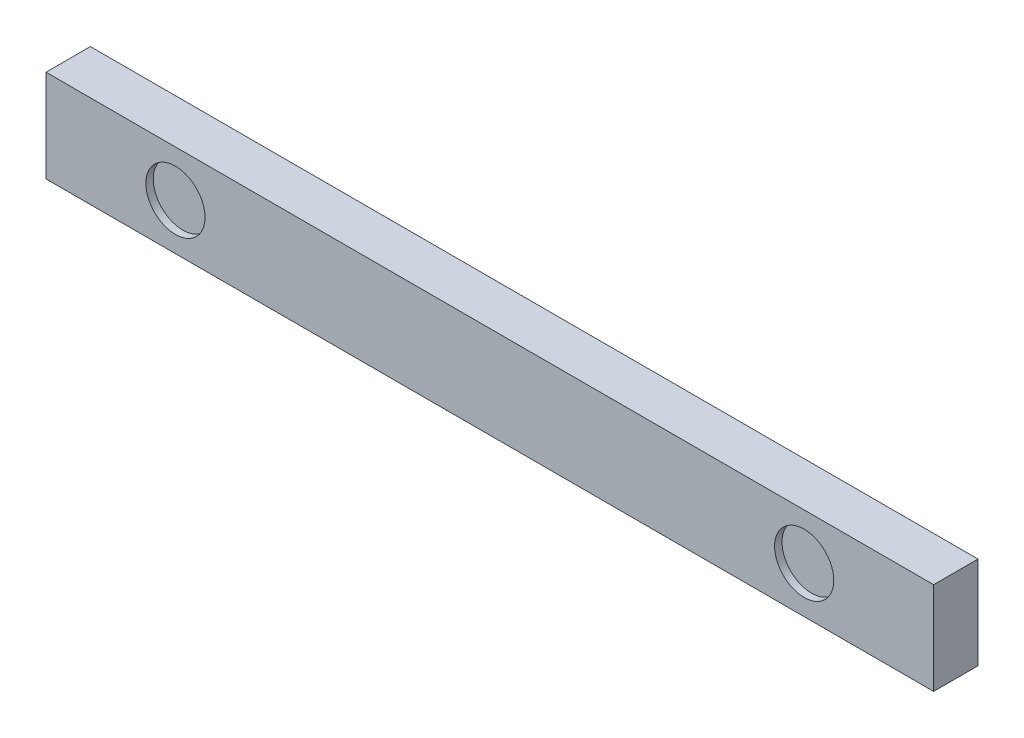
SolidWorks part; units mm, degrees
ref_plane "前视基准面" through (0, 0, 0) normal (0, 0, 1) x (1, 0, 0)
ref_plane "上视基准面" through (0, 0, 0) normal (0, 1, 0) x (1, 0, 0)
ref_plane "右视基准面" through (0, 0, 0) normal (1, 0, 0) x (0, 0, -1)
sketch "草图1" plane through (0, 0, 0) normal (0, 0, 1) x (1, 0, 0)
  line L1 (-120, -12.5) -> (120, -12.5)
  line L2 (-120, -12.5) -> (-120, 12.5)
  line L3 (-120, 12.5) -> (120, 12.5)
  line L4 (120, -12.5) -> (120, 12.5)
  line L5 (-120, -12.5) -> (120, 12.5) construction
  line L6 (-120, 12.5) -> (120, -12.5) construction
  point P0 (0, 0)
  dimension "D1" = 25
  dimension "D2" = 240
extrude "凸台-拉伸1" add sketch "草图1" along normal blind 12
sketch "草图2" plane through (0, 0, 12) normal (0, 0, 1) x (1, 0, 0)
  circle A0 centre (0, 0) radius 10.5 construction
  circle A1 centre (85, 0) radius 8
  circle A2 centre (-85, 0) radius 8
extrude "切除-拉伸1" cut sketch "草图2" against normal blind 2
equation "\"D5@草图2\"=\"D4@草图2\""
